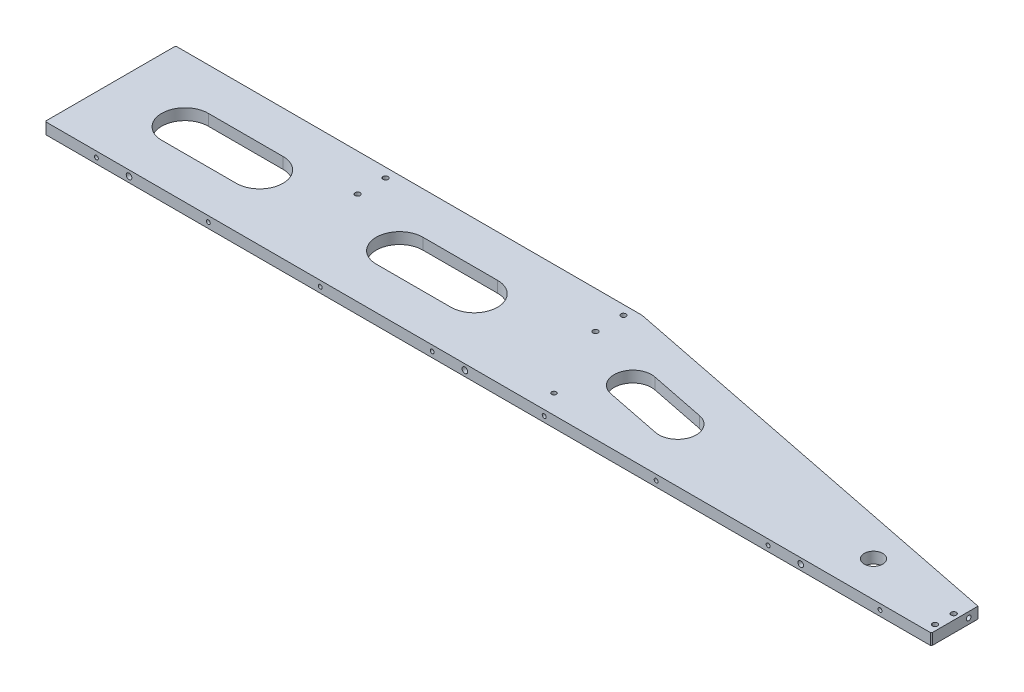
SolidWorks part; units mm, degrees
material "A7075"
ref_plane "Front Plane" through (0, 0, 0) normal (0, 0, 1) x (1, 0, 0)
ref_plane "Top Plane" through (0, 0, 0) normal (0, 1, 0) x (1, 0, 0)
ref_plane "Right Plane" through (0, 0, 0) normal (1, 0, 0) x (0, 0, -1)
sketch "Sketch2" plane through (0, 0, 0) normal (0, -1, 0) x (-1, 0, 0)
  line L0 (0, 0) -> (0, 140)
  line L1 (0, 140) -> (-500, 140)
  line L2 (-500, 140) -> (-950, 50)
  line L3 (-950, 50) -> (-950, 0)
  line L6 (0, 0) -> (-950, 0)
  dimension "D1" = 950
  dimension "D2" = 500
  dimension "D3" = 50
  dimension "D4" = 140
extrude "Boss-Extrude2" add sketch "Sketch2" against normal blind 12 separate body
sketch "Sketch9" plane through (0, 0, 0) normal (0, -1, 0) x (1, 0, 0)
  line L0 (80, -70) -> (160, -70) construction
  line L1 (80, -45) -> (160, -45)
  line L2 (80, -95) -> (160, -95)
  line L3 (310, -70) -> (390, -70) construction
  line L4 (310, -45) -> (390, -45)
  line L5 (310, -95) -> (390, -95)
  line L8 (950, -50) -> (950, 0) construction
  line L9 (560, -70) -> (620, -58) construction
  line L10 (556.0777, -50.3884) -> (616.0777, -38.3884)
  line L11 (563.9223, -89.6116) -> (623.9223, -77.6116)
  line L14 (950, 0) -> (0, 0) construction
  line L15 (0, 0) -> (0, -140) construction
  line L16 (500, -140) -> (950, -50) construction
  arc A0 (80, -45) -> (80, -95) centre (80, -70) ccw
  arc A1 (160, -95) -> (160, -45) centre (160, -70) ccw
  arc A2 (310, -45) -> (310, -95) centre (310, -70) ccw
  arc A3 (390, -95) -> (390, -45) centre (390, -70) ccw
  circle A4 centre (850, -38) radius 10
  arc A5 (556.0777, -50.3884) -> (563.9223, -89.6116) centre (560, -70) ccw
  arc A6 (623.9223, -77.6116) -> (616.0777, -38.3884) centre (620, -58) ccw
  point P2 (120, -70)
  point P7 (350, -70)
  point P24 (590, -64)
  dimension "D3" = 150
  dimension "D4" = 70
  dimension "D5" = 80
  dimension "D6" = 20
  dimension "D7" = 38
  dimension "D8" = 100
  dimension "D9" = 250
  dimension "D12" = 40
  dimension "D1" = 50
  dimension "D2" = 80
  dimension "D10" = 70
  dimension "D11" = 60
extrude "Cut-Extrude3" cut sketch "Sketch9" against normal blind 12
hole_wizard "M4 Tapped Hole2" positions "Sketch16" profile "Sketch15" tap size "M4" standard "Gb"
sketch "Sketch16" plane through (0, 0, 0) normal (0, -1, 0) x (-1, 0, 0)
  line L2 (0, 0) -> (0, 140) construction
  line L3 (-950, 0) -> (0, 0) construction
  circle A0 centre (-850, 38) radius 10 construction
  point P0 (-275, 10)
  point P2 (-275, 30)
  point P9 (-795, 23)
  point P11 (-905, 23)
  point P13 (-795, 53)
  point P15 (-905, 53)
  dimension "D6" = 55
  dimension "D7" = 15
  dimension "D1" = 20
  dimension "D2" = 275
  dimension "D3" = 10
  dimension "D4" = 30
  dimension "D5" = 110
sketch "Sketch15" plane through (275, 0, -10) normal (1, 0, 0) x (0, 0, -1)
  line L0 (0, 0) -> (0, 11.0914)
  line L1 (0, 11.0914) -> (1.65, 10.1)
  line L2 (1.65, 10.1) -> (1.65, 0)
  line L5 (1.65, 0) -> (0, 0)
  line L10 (0, 11.0914) -> (-1.65, 10.1) construction
  line L11 (0, -6.35) -> (0, 107.95) construction
  dimension "螺纹孔钻头直径" = 3.3
  dimension "螺纹孔钻头深度" = 10.1
  dimension "导头角度" = 118
cosmetic thread "Cosmetic thread 4" parameters "D1"=8, "D2"=4
cosmetic thread "Cosmetic thread 6" parameters "D1"=8, "D2"=4
cosmetic thread "Cosmetic thread 7" parameters "D1"=8, "D2"=4
cosmetic thread "Cosmetic thread 8" parameters "D1"=8, "D2"=4
cosmetic thread "Cosmetic thread 9" parameters "D1"=8, "D2"=4
cosmetic thread "Cosmetic thread 24" parameters "D1"=8, "D2"=4
hole_wizard "M6 Tapped Hole1" positions "Sketch14" profile "Sketch13" tap size "M6" standard "Gb"
sketch "Sketch14" plane through (0, 0, 0) normal (0, -1, 0) x (-1, 0, 0)
  line L1 (-950, 0) -> (0, 0) construction
  circle A1 centre (-275, 30) radius 1.65 construction
  point P0 (-525, 20.5)
  dimension "D1" = 20.5
  dimension "D2" = 250
sketch "Sketch13" plane through (525, 0, -20.5) normal (1, 0, 0) x (0, 0, -1)
  line L0 (0, 0) -> (0, 16.5022)
  line L1 (0, 16.5022) -> (2.5, 15)
  line L2 (2.5, 15) -> (2.5, 0)
  line L5 (2.5, 0) -> (0, 0)
  line L10 (0, 16.5022) -> (-2.5, 15) construction
  line L11 (0, -6.35) -> (0, 107.95) construction
  dimension "螺纹孔钻头直径" = 5
  dimension "螺纹孔钻头深度" = 15
  dimension "导头角度" = 118
cosmetic thread "Cosmetic thread 3" parameters "D1"=10, "D2"=6
hole_wizard "M4 Tapped Hole3" positions "Sketch25" profile "Sketch24" tap size "M4" standard "Gb"
sketch "Sketch25" plane through (0, 0, -140) normal (0, 0, -1) x (-1, 0, 0)
  line L1 (0, 0) -> (-500, 0) construction
  line L2 (0, 12) -> (0, 0) construction
  point P0 (-50, 6)
  point P4 (-400, 6)
  dimension "D1" = 50
  dimension "D2" = 350
  dimension "D4" = 6
sketch "Sketch24" plane through (50, 6, -140) normal (1, 0, 0) x (0, 1, 0)
  line L0 (0, 0) -> (0, 12.4914)
  line L1 (0, 12.4914) -> (1.65, 11.5)
  line L2 (1.65, 11.5) -> (1.65, 0)
  line L5 (1.65, 0) -> (0, 0)
  line L10 (0, 12.4914) -> (-1.65, 11.5) construction
  line L11 (0, -6.35) -> (0, 107.95) construction
  dimension "螺纹孔钻头直径" = 3.3
  dimension "螺纹孔钻头深度" = 11.5
  dimension "导头角度" = 118
cosmetic thread "Cosmetic thread 15" parameters "D1"=8, "D2"=4
cosmetic thread "Cosmetic thread 17" parameters "D1"=8, "D2"=4
hole_wizard "M4 Tapped Hole4" positions "Sketch27" profile "Sketch26" tap size "M4" standard "Gb"
sketch "Sketch27" plane through (46.1538, 0, -230.7692) normal (0.1961, 0, -0.9806) x (-0.9806, 0, -0.1961)
  line L0 (-462.8341, 0) -> (-921.7458, 0) construction
  line L2 (-921.7458, 12) -> (-921.7458, 0) construction
  point P4 (-871.7458, 6)
  point P6 (-521.7458, 6)
  dimension "D1" = 50
  dimension "D2" = 350
  dimension "D3" = 6
sketch "Sketch26" plane through (900.971, 6, -59.8058) normal (0, 1, 0) x (-0.9806, 0, -0.1961)
  line L0 (0, 0) -> (0, 12.4914)
  line L1 (0, 12.4914) -> (1.65, 11.5)
  line L2 (1.65, 11.5) -> (1.65, 0)
  line L5 (1.65, 0) -> (0, 0)
  line L10 (0, 12.4914) -> (-1.65, 11.5) construction
  line L11 (0, -6.35) -> (0, 107.95) construction
  dimension "螺纹孔钻头直径" = 3.3
  dimension "螺纹孔钻头深度" = 11.5
  dimension "导头角度" = 118
cosmetic thread "Cosmetic thread 18" parameters "D1"=8, "D2"=4
cosmetic thread "Cosmetic thread 19" parameters "D1"=8, "D2"=4
hole_wizard "M6 Tapped Hole3" positions "Sketch29" profile "Sketch28" tap size "M6" standard "Gb"
sketch "Sketch29" plane through (950, 0, 0) normal (1, 0, 0) x (0, 0, -1)
  line L0 (50, 0) -> (0, 0) construction
  line L1 (50, 12) -> (50, 0) construction
  point P0 (40, 6)
  point P2 (40, 96)
  dimension "D1" = 90
  dimension "D2" = 6
  dimension "D3" = 10
sketch "Sketch28" plane through (950, 6, -40) normal (0, 1, 0) x (0, 0, -1)
  line L0 (0, 0) -> (0, 18.5022)
  line L1 (0, 18.5022) -> (2.5, 17)
  line L2 (2.5, 17) -> (2.5, 0)
  line L5 (2.5, 0) -> (0, 0)
  line L10 (0, 18.5022) -> (-2.5, 17) construction
  line L11 (0, -6.35) -> (0, 107.95) construction
  dimension "螺纹孔钻头直径" = 5
  dimension "螺纹孔钻头深度" = 17
  dimension "导头角度" = 118
cosmetic thread "Cosmetic thread 23" parameters "D1"=12, "D2"=6
hole_wizard "M6 Tapped Hole2" positions "Sketch31" profile "Sketch30" tap size "M6" standard "Iso"
sketch "Sketch31" plane through (0, 0, 0) normal (-1, 0, 0) x (0, 0, 1)
  line L0 (-15, 6) -> (0, 6) construction
  line L1 (0, 12) -> (0, 0) construction
  point P0 (-15, 6)
  point P2 (-70, 6)
  point P4 (-125, 6)
  dimension "D1" = 110
  dimension "D2" = 15
  dimension "D3" = 55
sketch "Sketch30" plane through (0, 6, -15) normal (0, 1, 0) x (0, 0, 1)
  line L0 (0, 0) -> (0, 24.5022)
  line L1 (0, 24.5022) -> (2.5, 23)
  line L2 (2.5, 23) -> (2.5, 0)
  line L5 (2.5, 0) -> (0, 0)
  line L10 (0, 24.5022) -> (-2.5, 23) construction
  line L11 (0, -6.35) -> (0, 107.95) construction
  dimension "螺纹孔钻头直径" = 5
  dimension "螺纹孔钻头深度" = 23
  dimension "导头角度" = 118
cosmetic thread "Cosmetic thread 25" parameters "D1"=20, "D2"=6
cosmetic thread "Cosmetic thread 26" parameters "D1"=20, "D2"=6
cosmetic thread "Cosmetic thread 27" parameters "D1"=20, "D2"=6
hole_wizard "Ø6.0 (6) Diameter Hole1" positions "Sketch33" profile "Sketch32" hole size "Ø6.0" standard "Gb"
sketch "Sketch33" plane through (0, 0, 0) normal (-1, 0, 0) x (0, 0, 1)
  line L1 (0, 12) -> (0, 0) construction
  circle A0 centre (-70, 6) radius 2.5 construction
  point P0 (-30, 6)
  point P2 (-110, 6)
  point P9 (0, 6)
  dimension "D1" = 80
  dimension "D2" = 40
sketch "Sketch32" plane through (0, 6, -30) normal (0, 1, 0) x (0, 0, 1)
  line L0 (0, 0) -> (0, 16.8026)
  line L1 (0, 16.8026) -> (3, 15)
  line L2 (3, 15) -> (3, 0)
  line L5 (3, 0) -> (0, 0)
  line L10 (0, 16.8026) -> (-3, 15) construction
  line L11 (0, -6.35) -> (0, 107.95) construction
  dimension "孔直径" = 6
  dimension "孔深度" = 15
  dimension "导头角度" = 118
hole_wizard "M5 Tapped Hole1" positions "Sketch36" profile "Sketch34" tap size "M5" standard "Iso"
sketch "Sketch36" plane through (0, 0, 0) normal (0, 0, 1) x (1, 0, 0)
  line L0 (0, 6) -> (1106.8343, 6) construction
  line L1 (0, 12) -> (0, 0) construction
  point P0 (55, 6)
  point P10 (175, 6)
  point P12 (295, 6)
  point P14 (415, 6)
  point P16 (535, 6)
  point P18 (655, 6)
  point P20 (775, 6)
  point P22 (895, 6)
  dimension "D3" = 120
  dimension "D4" = 120
  dimension "D5" = 120
  dimension "D6" = 120
  dimension "D7" = 120
  dimension "D8" = 120
  dimension "D9" = 120
  dimension "D10" = 55
sketch "Sketch34" plane through (55, 6, 0) normal (1, 0, 0) x (0, -1, 0)
  line L0 (0, 0) -> (0, 13.6618)
  line L1 (0, 13.6618) -> (2.1, 12.4)
  line L2 (2.1, 12.4) -> (2.1, 0)
  line L5 (2.1, 0) -> (0, 0)
  line L10 (0, 13.6618) -> (-2.1, 12.4) construction
  line L11 (0, -6.35) -> (0, 107.95) construction
  dimension "螺纹孔钻头直径" = 4.2
  dimension "螺纹孔钻头深度" = 12.4
  dimension "导头角度" = 118
cosmetic thread "Cosmetic thread 30" parameters "D1"=10, "D2"=5
cosmetic thread "Cosmetic thread 31" parameters "D1"=10, "D2"=5
cosmetic thread "Cosmetic thread 32" parameters "D1"=10, "D2"=5
cosmetic thread "Cosmetic thread 33" parameters "D1"=10, "D2"=5
cosmetic thread "Cosmetic thread 34" parameters "D1"=10, "D2"=5
cosmetic thread "Cosmetic thread 35" parameters "D1"=10, "D2"=5
cosmetic thread "Cosmetic thread 36" parameters "D1"=10, "D2"=5
cosmetic thread "Cosmetic thread 37" parameters "D1"=10, "D2"=5
hole_wizard "Ø6.0 (6) Diameter Hole2" positions "Sketch38" profile "Sketch37" hole size "Ø6.0" standard "Gb"
sketch "Sketch38" plane through (0, 0, 0) normal (0, 0, 1) x (1, 0, 0)
  line L0 (0, 12) -> (0, 0) construction
  point P0 (90, 6)
  point P2 (450, 6)
  point P4 (810, 6)
  point P13 (0, 6)
  dimension "D1" = 90
  dimension "D2" = 360
  dimension "D3" = 360
sketch "Sketch37" plane through (90, 6, 0) normal (1, 0, 0) x (0, -1, 0)
  line L0 (0, 0) -> (0, 16.8026)
  line L1 (0, 16.8026) -> (3, 15)
  line L2 (3, 15) -> (3, 0)
  line L5 (3, 0) -> (0, 0)
  line L10 (0, 16.8026) -> (-3, 15) construction
  line L11 (0, -6.35) -> (0, 107.95) construction
  dimension "孔直径" = 6
  dimension "孔深度" = 15
  dimension "导头角度" = 118
hole_wizard "Hole size per hex socket screw type1" positions "Sketch40" profile "Sketch39" counterbore size "M5" standard "Gb" end condition through all
sketch "Sketch40" plane through (0, 0, 0) normal (0, -1, 0) x (-1, 0, 0)
  line L0 (0, 140) -> (-500, 140) construction
  line L1 (0, 0) -> (0, 140) construction
  line L2 (-950, 50) -> (-950, 0) construction
  line L3 (-950, 0) -> (0, 0) construction
  point P0 (-235, 100)
  point P2 (-235, 130)
  point P4 (-490, 100)
  point P6 (-490, 130)
  point P8 (-944, 10)
  point P10 (-944, 30)
  dimension "D1" = 30
  dimension "D2" = 10
  dimension "D3" = 235
  dimension "D4" = 255
  dimension "D5" = 6
  dimension "D6" = 10
  dimension "D7" = 20
sketch "Sketch39" plane through (235, 0, -100) normal (1, 0, 0) x (0, 0, -1)
  line L0 (0, 0) -> (0, 12)
  line L1 (0, 12) -> (2.75, 12)
  line L3 (2.75, 12) -> (2.75, 5.7)
  line L4 (2.75, 5.7) -> (5, 5.7)
  line L5 (5, 5.7) -> (5, 0)
  line L7 (5, 0) -> (0, 0)
  line L11 (0, -6.35) -> (0, 107.95) construction
  dimension "通孔孔直径" = 5.5
  dimension "通孔孔深度" = 12
  dimension "柱形沉头孔直径" = 10
  dimension "柱形沉头孔深度" = 5.7
chamfer "Chamfer2" distance 1 angle 45 3 edges at (0, 6, -140) (0, 6, 0) (950, 6, 0)
